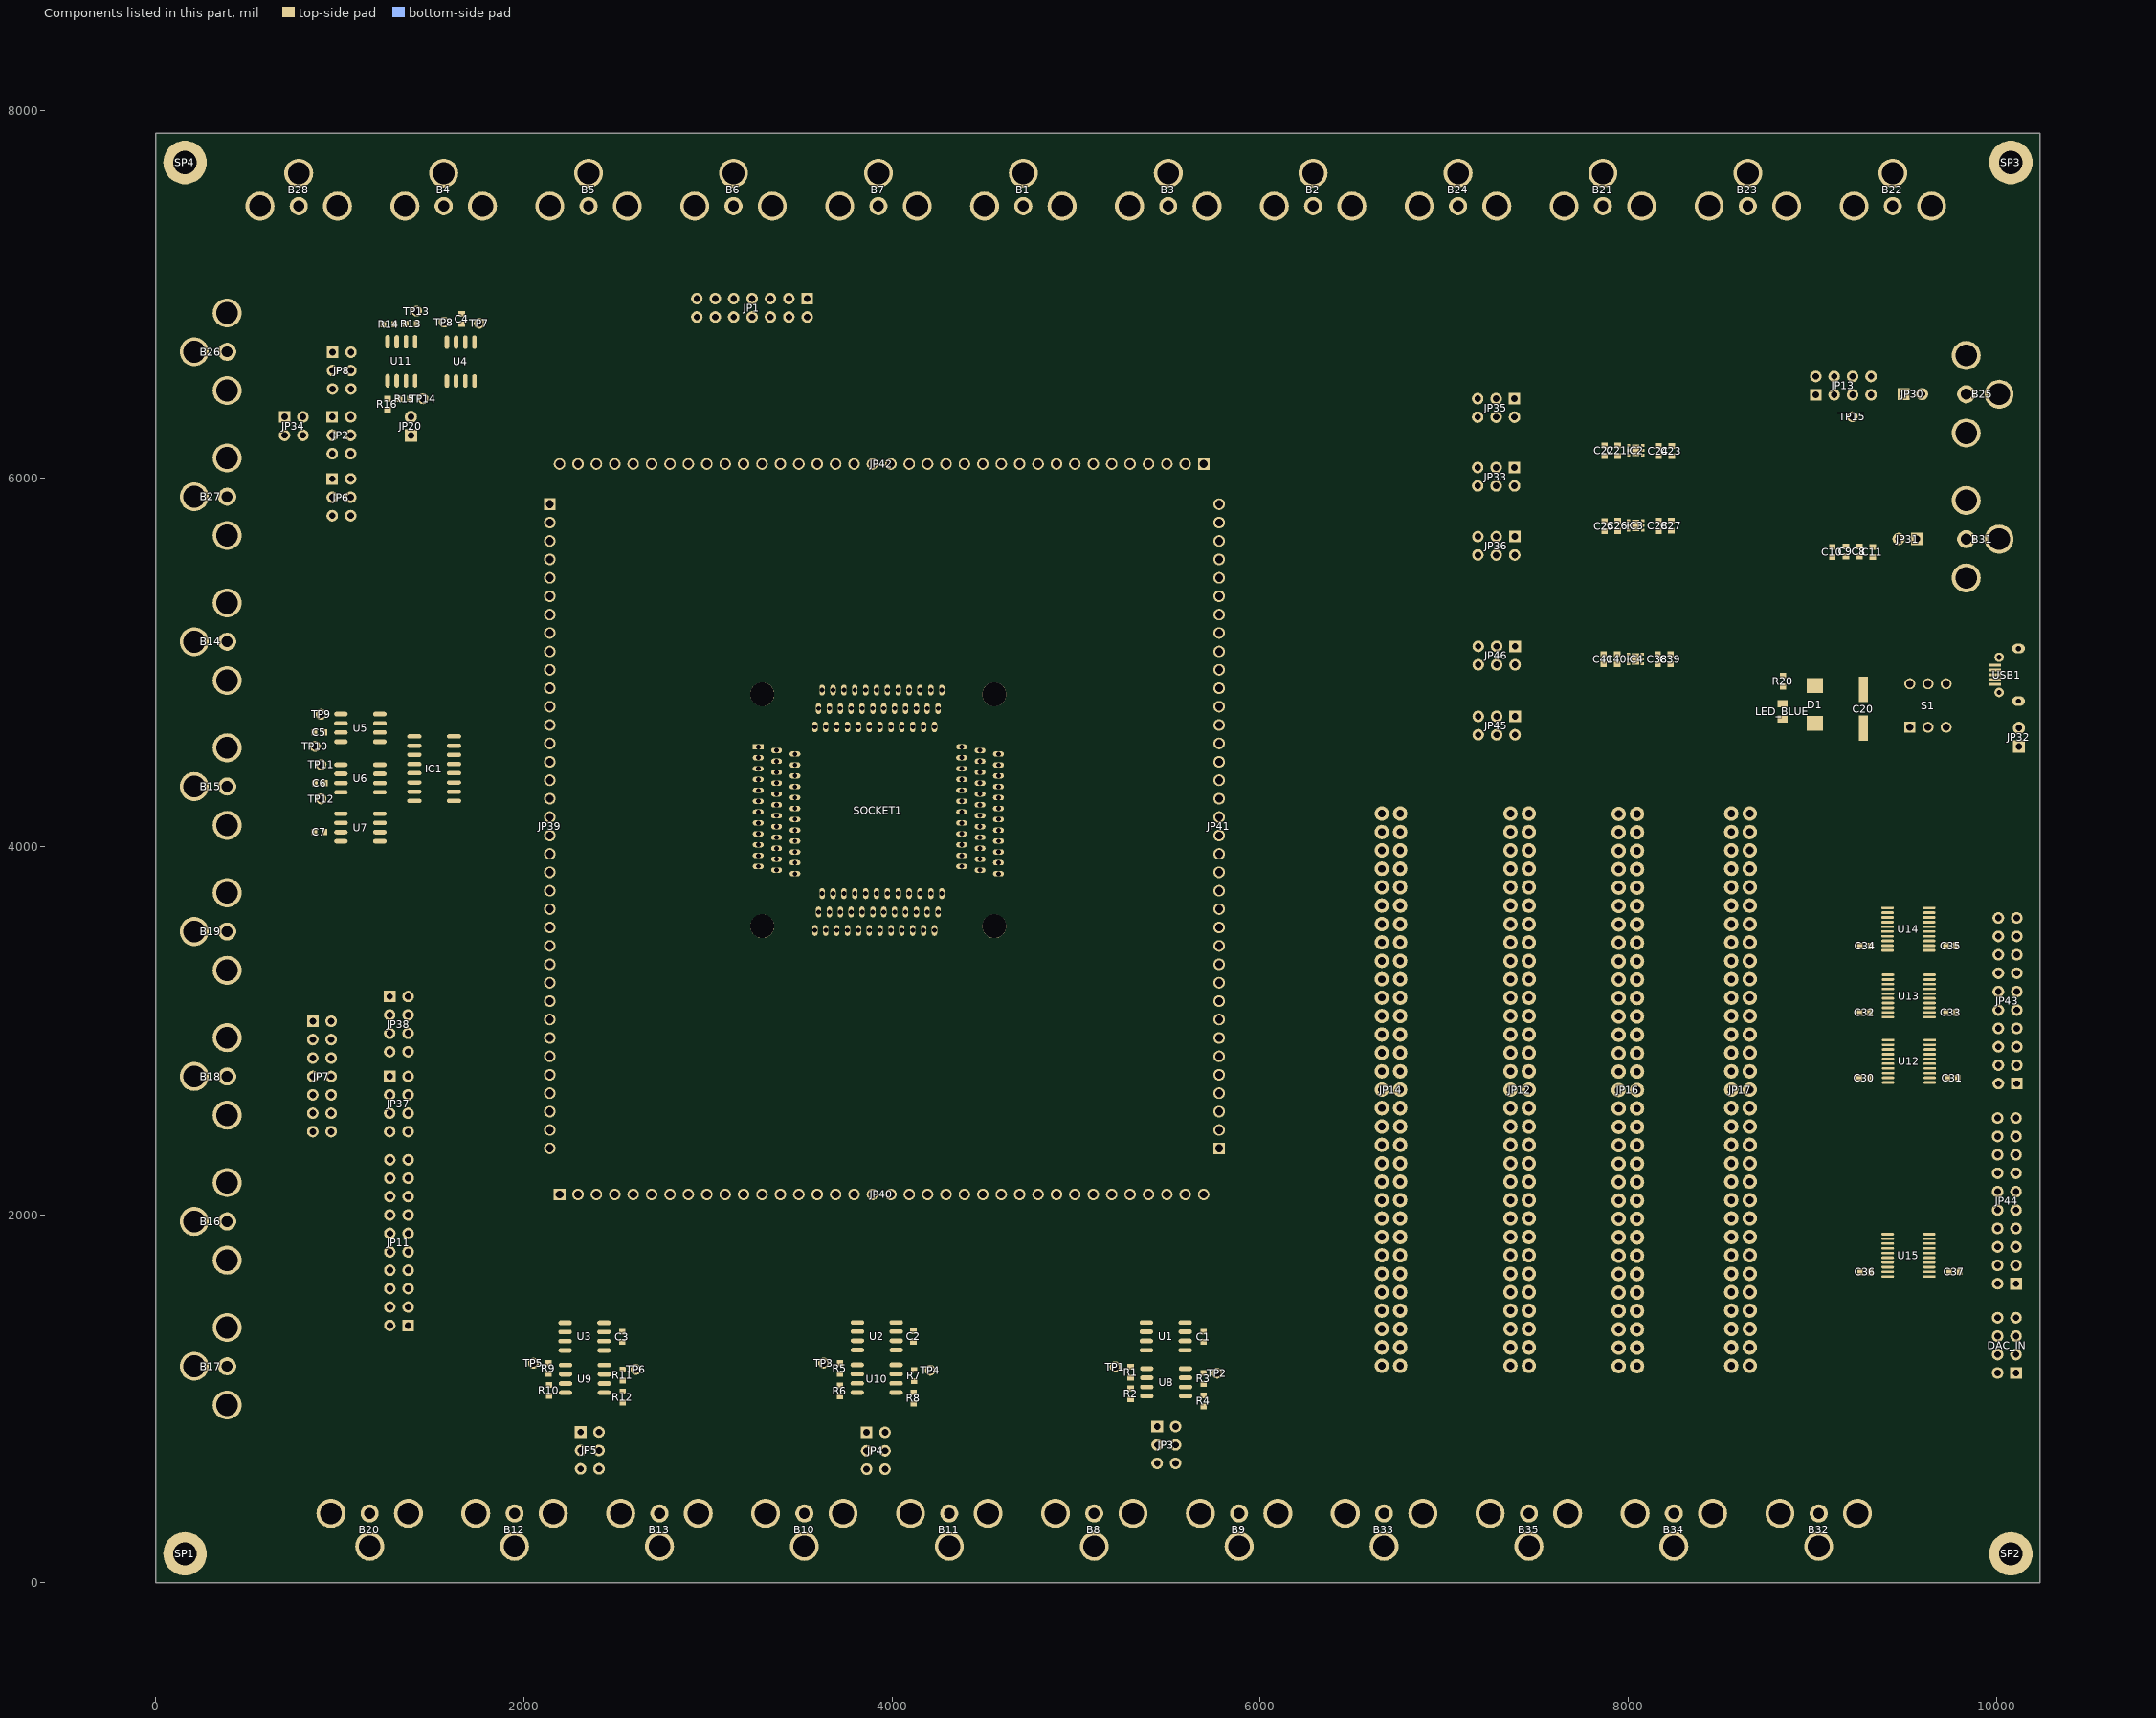
[diagram p0: the components of this part, seen from the top]
# Altium PCB MISC62794.PcbDoc (part 7 of 7)
Units mil, origin at the board's own origin, x right, y up, seen from the top; angles counter-clockwise.
Board outline 10236.22 x 7874.02 mil, 4 copper layers (Top Layer, GND, POWER, Bottom Layer); 158 components, 185 nets, 1211 pads, 1759 vias.

## Silkscreen, mask and mechanical layers (free items; w line width, h text height)
Top Overlay:
  text "VSSH" at 6229,7339 h50
  text "VBIT_PS_OUT2" at 7697,7338 h50
  text "VG_PS_OUT" at 9297,7336 h50
  text "VS_PS_OUT" at 8518,7335 h50
  text "VDD" at 3108,7334 h50
  text "VDDH" at 4647,7334 h50
  text "VDDC" at 5433,7334 h50
  text "VDD25" at 2297,7333 h50
  text "VBIT_PS_OUT1" at 6929,7328 h50
  text "VSS" at 3877,7317 h50
  text "VSSC" at 1511,7309 h50
  text "GND" at 730,7308 h50
  text "DAC14" at 782,6675 h40
  text "V25" at 528,6651 h50 r90
  text "GND" at 9233,6617 h40 r90
  text "GND" at 9132,6616 h40 r90
  text "GND" at 9334,6616 h40 r90
  text "GND" at 9028,6615 h40 r90
  text "FORMING" at 738,6570 h40
  text "GND" at 7245,6508 h40
  text "GND" at 7351,6507 h40
  text "GND" at 7145,6506 h40
  text "V25" at 832,6474 h40
  text "DCDC_OUT" at 9718,6332 h50 r90
  text "V25" at 1128,6311 h40
  text "V25" at 1209,6310 h40
  text "USB_5V" at 9032,6260 h40 r90
  text "USB_5V" at 9133,6257 h40 r90
  text "V11" at 7142,6242 h40
  text "V25" at 7247,6241 h40
  text "VCC5V" at 7346,6241 h40
  text "V11" at 1133,6219 h40
  text "V11" at 1234,6217 h40
  text "TEST" at 9233,6206 h40 r90
  text "DCDC_OUT" at 9333,6198 h40 r90
  text "VS1" at 3608,6169 h40 r90
  text "TSETDELAY_IN" at 3510,6168 h40 r90
  text "IREF" at 4006,6167 h40 r90
  text "TEST_PS_CTRL" at 3407,6166 h40 r90
  text "VSSC" at 3308,6165 h40 r90
  text "VLIM" at 3908,6165 h40 r90
  text "VS2" at 3712,6164 h40 r90
  text "VS_PS_OUT" at 4906,6164 h40 r90
  text "VDD" at 4408,6163 h40 r90
  text "VRES" at 3802,6162 h40 r90
  text "VSS" at 4304,6162 h40 r90
  text "VDDH" at 4604,6162 h40 r90
  text "VDDC" at 4709,6161 h40 r90
  text "VDDC" at 3204,6160 h40 r90
  text "VBIT_PS_OUT1" at 4109,6160 h40 r90
  text "VDD25" at 4505,6160 h40 r90
  text "NC" at 5706,6160 h40 r90
  text "VBIT_PS_OUT2" at 4207,6159 h40 r90
  text "VDDH" at 4806,6159 h40 r90
  text "CSB_ADD_1" at 5604,6156 h40 r90
  text "VDDH" at 3106,6155 h40 r90
  text "NC" at 2203,6154 h40 r90
  text "VBIT1" at 2402,6154 h40 r90
  text "VSSC" at 5208,6154 h40 r90
  text "CSB_ADD_4" at 5503,6153 h40 r90
  text "VSSH" at 2301,6152 h40 r90
  text "VBIT2" at 2508,6152 h40 r90
  text "VBIT_PS_CTRL" at 2806,6151 h40 r90
  text "VG_PS_CTRL" at 2905,6151 h40 r90
  text "VS_PS_CTRL" at 3006,6151 h40 r90
  text "CSB_ADD_2" at 5103,6150 h40 r90
  text "VG1" at 2606,6149 h40 r90
  text "CSB_ADD_0" at 5401,6149 h40 r90
  text "VG_PS_OUT" at 5011,6148 h40 r90
  text "VG2" at 2706,6147 h40 r90
  text "CSB_ADD_3" at 5303,6147 h40 r90
  text "GND" at 7245,6135 h40
  text "GND" at 7351,6134 h40
  text "GND" at 7145,6133 h40
  text "GND" at 1126,6118 h40
  text "GND" at 1222,6117 h40
  text "GND" at 821,5992 h40
  text "GND" at 1137,5991 h40
  text "GND" at 1138,5887 h40
  text "GND" at 816,5886 h40
  text "V11" at 523,5865 h50 r90
  text "V11" at 7145,5861 h40
  text "V25" at 7250,5860 h40
  text "VCC5V" at 7349,5860 h40
  text "NC" at 5924,5854 h40
  text "NC" at 1975,5851 h40
  text "NC" at 834,5786 h40
  text "NC" at 1143,5785 h40
  text "GND" at 7253,5757 h40
  text "GND" at 7359,5756 h40
  text "NC" at 1971,5755 h40
  text "GND" at 7153,5755 h40
  text "NC" at 5924,5747 h40
  text "NC" at 1967,5647 h40
  text "NC" at 5929,5646 h40
  text "VCC_5V" at 9711,5590 h50 r90
  text "NC" at 1966,5549 h40
  text "NC" at 5931,5546 h40
  text "V11" at 7147,5484 h40
  text "V25" at 7252,5483 h40
  text "VCC5V" at 7351,5483 h40
  text "NC" at 5934,5444 h40
  text "NC" at 1965,5443 h40
  text "NC" at 5938,5348 h40
  text "NC" at 1964,5347 h40
  text "Vbit_0" at 1903.04,5255 h40
  text "Vbit_16" at 5940.68,5248 h40
  text "GND" at 7254,5162 h40
  text "GND" at 7360,5161 h40
  text "GND" at 7154,5160 h40
  text "Vbit_1" at 1903.04,5150 h40
  text "Vbit_19" at 5940.6,5146 h40
  text "Vbit_2" at 1903.04,5055 h40
  text "VLIM" at 533,5054 h50 r90
  text "Vbit_17" at 5940.68,5049 h40
  text "Vbit_3" at 1903.04,4947 h40
  text "Vbit_22" at 5940.91,4946 h40
  text "3V3" at 7148,4887 h40
  text "3V3" at 7253,4886 h40
  text "VCC5V" at 7352,4886 h40
  text "Vbit_4" at 1903.04,4854 h40
  text "Vbit_20" at 5940.76,4849 h40
  text "GND" at 7249,4781 h40
  text "GND" at 7355,4780 h40
  text "GND" at 7149,4779 h40
  text "Vbit_5" at 1903.04,4751 h40
  text "Vbit_18" at 5940.6,4741 h40
  text "Vbit_6" at 1903.04,4653 h40
  text "Vbit_25" at 5940.48,4642 h40
  text "Vbit_7" at 1903.04,4556 h40
  text "Vbit_23" at 5940.68,4548 h40
  text "3V3" at 7156,4510 h40
  text "3V3" at 7261,4509 h40
  text "VCC5V" at 7360,4509 h40
  text "Vbit_8" at 1903.04,4454 h40
  text "Vbit_21" at 5945.59,4443 h40
  text "Vbit_9" at 1903.04,4357 h40
  text "VDDH" at 5961.94,4345 h40
  text "IREF" at 536,4268 h50 r90
  text "Vbit_10" at 1903.04,4251 h40
  text "Vbit_24" at 5940.76,4244 h40
  text "Vbit_16" at 6449,4184 h40
  text "VF3" at 7535,4174 h40
  text "VF1" at 8738,4174 h40
  text "Vbit_16" at 7148,4173 h40
  text "VF4" at 6831,4172 h40
  text "VF2" at 8130,4171 h40
  text "Vbit_16" at 7750,4167 h40
  text "Vbit_16" at 8358,4162 h40
  text "Vbit_11" at 1903.04,4154 h40
  text "VDDC" at 5960.45,4146 h40
  text "Vbit_19" at 6449,4078 h40
  text "VF3" at 7535,4072 h40
  text "Vbit_19" at 7148,4067 h40
  text "VF4" at 6831,4066 h40
  text "VF2" at 8129,4065 h40
  text "VF1" at 8738,4065 h40
  text "Vbit_19" at 7750,4061 h40
  text "Vbit_19" at 8358,4056 h40
  text "Vbit_12" at 1903.04,4053 h40
  text "VSSH" at 5965.84,4048 h40
  text "Vbit_17" at 6449,3979 h40
  text "VF1" at 8738,3972 h40
  text "VF3" at 7535,3971 h40
  text "VF4" at 6831,3970 h40
  text "VF2" at 8132,3969 h40
  text "Vbit_17" at 7148,3968 h40
  text "Vbit_17" at 7750,3962 h40
  text "Vbit_17" at 8358,3957 h40
  text "VSSC" at 1903.04,3951 h40
  text "VSSC" at 5964.35,3945 h40
  text "Vbit_22" at 6449,3878 h40
  text "VF3" at 7535,3871 h40
  text "Vbit_22" at 7148,3867 h40
  text "VF4" at 6831,3866 h40
  text "VF2" at 8133,3865 h40
  text "VF1" at 8738,3864 h40
  text "Vbit_22" at 7750,3861 h40
  text "Vbit_22" at 8358,3856 h40
  text "VSSH" at 1903.04,3852 h40
  text "Vbit_26" at 5940.68,3848 h40
  text "VF3" at 7535,3777 h40
  text "Vbit_20" at 6449,3775 h40
  text "VF1" at 8738,3768 h40
  text "VF4" at 6831,3767 h40
  text "Vbit_20" at 7148,3764 h40
  text "VF2" at 8134,3764 h40
  text "Vbit_20" at 7750,3758 h40
  text "VDDC" at 1903.04,3753 h40
  text "Vbit_20" at 8358,3753 h40
  text "Vbit_27" at 5940.68,3749 h40
  text "Vbit_18" at 6449,3672 h40
  text "VF2" at 8136,3670 h40
  text "VF4" at 6831,3668 h40
  text "VF3" at 7535,3666 h40
  text "VF1" at 8738,3665 h40
  text "Vbit_18" at 7148,3661 h40
  text "Vbit_18" at 7750,3655 h40
  text "Vbit_18" at 8358,3650 h40
  text "Vbit_14" at 1903.04,3647 h40
  text "Vbit_28" at 5940.6,3645 h40
  text "VG5" at 9798,3604 h40
  text "VG4" at 9879,3601 h40
  text "VF3" at 7542,3574 h40
  text "VF1" at 8737,3570 h40
  text "Vbit_25" at 6449,3569 h40
  text "VF4" at 6832,3568 h40
  text "VF2" at 8135,3564 h40
  text "Vbit_25" at 7148,3558 h40
  text "Vbit_25" at 7750,3552 h40
  text "Vbit_25" at 8358,3547 h40
  text "Vbit_29" at 5940.6,3546 h40
  text "VDDH" at 1903.04,3544 h40
  text "VG2" at 9880,3506 h40
  text "VG3" at 9797,3505 h40
  text "VRES" at 541,3491 h50 r90
  text "VF3" at 7542,3472 h40
  text "Vbit_23" at 6449,3470 h40
  text "VF2" at 8138,3468 h40
  text "VF4" at 6832,3462 h40
  text "VF1" at 8737,3461 h40
  text "Vbit_23" at 7148,3459 h40
  text "Vbit_23" at 7750,3453 h40
  text "Vbit_23" at 8358,3448 h40
  text "Vs_Sel_1" at 1903.04,3447 h40
  text "Vbit_30" at 5940.76,3446 h40
  text "VG0" at 9876,3403 h40
  text "VG1" at 9796,3401 h40
  text "Vbit_21" at 6449,3372 h40
  text "VF3" at 7542,3371 h40
  text "VF1" at 8737,3368 h40
  text "VF4" at 6832,3366 h40
  text "VF2" at 8139,3364 h40
  text "Vbit_21" at 7148,3361 h40
  text "Vbit_21" at 7750,3355 h40
  text "READ_EN" at 5897,3351 h40
  text "Vbit_21" at 8358,3350 h40
  text "WL_TEST" at 1903,3343 h40
  text "VS4" at 9882,3312 h40
  text "VS5" at 9797,3307 h40
  text "Vbit_24" at 6449,3271 h40
  text "VF3" at 7542,3271 h40
  text "STROBE" at 5916.7,3263 h40
  text "VF2" at 8140,3263 h40
  text "VF4" at 6832,3262 h40
  text "Vbit_24" at 7148,3260 h40
  text "VF1" at 8737,3260 h40
  text "Vbit_24" at 7750,3254 h40
  text "Vbit_13" at 1903.04,3250 h40
  text "Vbit_24" at 8358,3249 h40
  text "VS2" at 9884,3212 h40
  text "VS3" at 9793,3208 h40
  text "GND" at 1551,3180 h40
  text "VF3" at 7542,3177 h40
  text "V11" at 1446,3175 h40
  text "Vbit_26" at 6449,3170 h40
  text "VF1" at 8737,3164 h40
  text "VF4" at 6832,3163 h40
  text "Vbit_26" at 7148,3159 h40
  text "VF2" at 8140,3154 h40
  text "Vbit_26" at 7750,3153 h40
  text "Vbit_26" at 8358,3148 h40
  text "OEN" at 5987.36,3147 h40
  text "Vs_Sel_2" at 1903.04,3144 h40
  text "VS1" at 9815,3099 h40
  text "VS0" at 9889,3099 h40
  text "GND" at 1555,3077 h40
  text "Vbit_27" at 6449,3077 h40
  text "VLIM" at 1440,3074 h40
  text "Vbit_27" at 7148,3066 h40
  text "VF3" at 7542,3066 h40
  text "VF4" at 6832,3064 h40
  text "VF1" at 8737,3061 h40
  text "Vbit_27" at 7750,3060 h40
  text "Vbit_27" at 8358,3055 h40
  text "STATE_1" at 5913.34,3054 h40
  text "Vs_Sel_0" at 1903.04,3052 h40
  text "VF2" at 8139,3048 h40
  text "VLIM" at 691,3045 h40
  text "DAC7" at 1021,3043 h40
  text "STATE1" at 9815,2992 h40
  text "STATE2" at 9664,2991 h40
  text "GND" at 1558,2981 h40
  text "IREF" at 1446,2977 h40
  text "VF3" at 7546,2972 h40
  text "VF1" at 8735,2968 h40
  text "Vbit_28" at 6449,2965 h40
  text "VF4" at 6832,2965 h40
  text "Vbit_28" at 7148,2954 h40
  text "Vs_Sel_3" at 1903.04,2953 h40
  text "VF2" at 8142,2952 h40
  text "STATE_0" at 5908.51,2949 h40
  text "Vbit_28" at 7750,2948 h40
  text "IREF" at 706,2944 h40
  text "Vbit_28" at 8358,2943 h40
  text "DAC8" at 1017,2942 h40
  text "STATE0" at 9693,2903 h40
  text "ADD4" at 9853,2901 h40
  text "Vbit_29" at 6449,2882 h40
  text "GND" at 1558,2877 h40
  text "VREF" at 1448,2875 h40
  text "Vbit_29" at 7148,2871 h40
  text "VF3" at 7546,2870 h40
  text "Vbit_29" at 7750,2865 h40
  text "Vbit_29" at 8358,2860 h40
  text "VF4" at 6832,2859 h40
  text "VF1" at 8735,2859 h40
  text "NC" at 2004,2851 h40
  text "VF2" at 8143,2848 h40
  text "NC" at 5921,2847 h40
  text "DAC9" at 1020,2843 h40
  text "VRES" at 689,2838 h40
  text "ADD3" at 9695,2804 h40
  text "ADD2" at 9845,2803 h40
  text "Vbit_30" at 6449,2774 h40
  text "VF3" at 7546,2769 h40
  text "VF1" at 8735,2766 h40
  text "VF4" at 6832,2763 h40
  text "Vbit_30" at 7148,2763 h40
  text "NC" at 5921,2758 h40
  text "Vbit_30" at 7750,2757 h40
  text "Vbit_30" at 8358,2752 h40
  text "NC" at 2007,2751 h40
  text "VF2" at 8144,2747 h40
  text "GND" at 1614,2745 h40
  text "VS_PS" at 1441,2742 h40
  text "DAC10" at 1018,2741 h40
  text "VS_PS" at 675,2736 h40
  text "ADD0" at 9852,2672 h40
  text "ADD1" at 9711,2671 h40
  text "VF3" at 7546,2669 h40
  text "Vbit_0" at 6449,2663 h40
  text "NC" at 5918,2662 h40
  text "VF2" at 8146,2662 h40
  text "VF4" at 6832,2659 h40
  text "VF1" at 8735,2658 h40
  text "NC" at 2009,2655 h40
  text "Vbit_0" at 7148,2652 h40
  text "Vbit_0" at 7750,2646 h40
  text "DAC11" at 1020,2641 h40
  text "Vbit_0" at 8358,2641 h40
  text "VBIT_PS" at 1438,2639 h40
  text "GND" at 1616,2639 h40
  text "VBIT_PS" at 644,2636 h40
  text "VS_PS_CTRL" at 546,2603 h50 r90
  text "VF3" at 7546,2575 h40
  text "Vbit_1" at 6449,2567 h40
  text "VF1" at 8735,2562 h40
  text "VF4" at 6832,2560 h40
  text "NC" at 5918,2558 h40
  text "Vbit_1" at 7148,2556 h40
  text "VF2" at 8145,2556 h40
  text "NC" at 2010,2551 h40
  text "Vbit_1" at 7750,2550 h40
  text "Vbit_1" at 8358,2545 h40
  text "DAC12" at 1024,2544 h40
  text "GND" at 1611,2540 h40
  text "VG_PS" at 1446,2538 h40
  text "VG_PS" at 664,2534 h40
  text "NC" at 9823,2517 h40
  text "NC" at 9713,2515 h40
  text "Vbit_2" at 6449,2464 h40
  text "VF3" at 7546,2464 h40
  text "VF4" at 6832,2461 h40
  text "VF2" at 8148,2460 h40
  text "VF1" at 8735,2459 h40
  text "NC" at 5918,2454 h40
  text "Vbit_2" at 7148,2453 h40
  text "NC" at 2009,2448 h40
  text "Vbit_2" at 7750,2447 h40
  text "Vbit_2" at 8358,2442 h40
  text "TEST_PS" at 631,2440 h40
  text "DAC13" at 1022,2440 h40
  text "TEST_PS" at 1444,2437 h40
  text "GND" at 1622,2437 h40
  text "NC" at 9827,2415 h40
  text "NC" at 9715,2408 h40
  text "VF3" at 7551,2368 h40
  text "VF1" at 8734,2368 h40
  text "Vbit_3" at 6449,2364 h40
  text "VF4" at 6837,2363 h40
  text "VF2" at 8149,2356 h40
  text "Vbit_3" at 7148,2353 h40
  text "NC" at 5918,2351 h40
  text "NC" at 2012,2349 h40
  text "Vbit_3" at 7750,2347 h40
  text "Vbit_3" at 8358,2342 h40
  text "NC" at 9829,2320 h40
  text "NC" at 9714,2316 h40
  text "NC" at 1121,2295 h40
  text "NC" at 1476,2292 h40
  text "VF3" at 7551,2266 h40
  text "Vbit_4" at 6449,2261 h40
  text "VF1" at 8734,2259 h40
  text "VF4" at 6837,2257 h40
  text "VF2" at 8150,2255 h40
  text "Vbit_4" at 7148,2250 h40
  text "Vbit_4" at 7750,2244 h40
  text "Vbit_4" at 8358,2239 h40
  text "NC" at 9834,2219 h40
  text "NC" at 9719,2213 h40
  text "NC" at 1122,2186 h40
  text "NC" at 1479,2186 h40
  text "VF1" at 8734,2166 h40
  text "Vbit_5" at 6449,2165 h40
  text "VF3" at 7551,2165 h40
  text "VF4" at 6837,2161 h40
  text "Vbit_5" at 7148,2154 h40
  text "VF2" at 8149,2151 h40
  text "Vbit_5" at 7750,2148 h40
  text "Vbit_5" at 8358,2143 h40
  text "NC" at 9716,2122 h40
  text "IN_MCU" at 9810,2121 h40
  text "GND" at 1106,2087 h40
  text "OUT5" at 1458,2086 h40
  text "Vbit_6" at 6449,2068 h40
  text "VF3" at 7551,2065 h40
  text "VF1" at 8734,2058 h40
  text "VF4" at 6837,2057 h40
  text "Vbit_6" at 7148,2057 h40
  text "Vbit_6" at 7750,2051 h40
  text "Vbit_6" at 8358,2046 h40
  text "VF2" at 8148,2045 h40
  text "WL_TEST_MCU" at 9468,2015 h40
  text "OEN_MCU" at 9770,2015 h40
  text "GND" at 1108,1991 h40
  text "OUT7" at 1455,1985 h40
  text "NC" at 2209,1977 h40 r90
  text "VF3" at 7551,1971 h40
  text "VF1" at 8734,1962 h40
  text "Vbit_7" at 6449,1961 h40
  text "VF4" at 6837,1958 h40
  text "Vbit_7" at 7148,1950 h40
  text "VF2" at 8151,1949 h40
  text "Vbit_7" at 7750,1944 h40
  text "Vbit_7" at 8358,1939 h40
  text "STROBE_MCU" at 9702,1928 h40
  text "READ_EN_MCU" at 9409,1927 h40
  text "NC" at 5702,1917 h40 r90
  text "OUT_0" at 5004,1915 h40 r90
  text "VDDH" at 5599,1908 h40 r90
  text "VSSC" at 4104,1906 h40 r90
  text "OUT_3" at 4601,1904 h40 r90
  text "OUT_1" at 4203,1902 h40 r90
  text "VDDH" at 4308,1902 h40 r90
  text "VDDC" at 4404,1902 h40 r90
  text "VSS" at 4004,1901 h40 r90
  text "OUT_4" at 3803,1900 h40 r90
  text "VDD" at 3706,1899 h40 r90
  text "VDD25" at 5501,1898 h40 r90
  text "OUT_2" at 3899,1896 h40 r90
  text "VSSH" at 5399,1896 h40 r90
  text "OUT_6" at 3604,1895 h40 r90
  text "VSSC" at 3112,1893 h40 r90
  text "OUT_7" at 3501,1892 h40 r90
  text "OUT_5" at 3404,1891 h40 r90
  text "Vs_Sel_4" at 2305,1889 h40 r90
  text "Vs_Sel_5" at 2400,1889 h40 r90
  text "VDDC" at 3009,1887 h40 r90
  text "VSSH" at 3305,1887 h40 r90
  text "GND" at 1109,1886 h40
  text "VG_Sel_0" at 2506,1886 h40 r90
  text "VG_Sel_4" at 2903,1886 h40 r90
  text "STATE_2" at 5102,1885 h40 r90
  text "VG_Sel_1" at 2602,1883 h40 r90
  text "VG_Sel_2" at 2701,1883 h40 r90
  text "VG_Sel_3" at 2800,1883 h40 r90
  text "VG_Sel_5" at 3204,1883 h40 r90
  text "STATE_1" at 5201,1883 h40 r90
  text "OUT6" at 1457,1882 h40
  text "Vbit_8" at 6449,1869 h40
  text "VF3" at 7551,1860 h40
  text "VF4" at 6837,1859 h40
  text "VF1" at 8734,1859 h40
  text "Vbit_8" at 7148,1858 h40
  text "VBIT_Sel_2" at 4501,1853 h40 r90
  text "Vbit_8" at 7750,1852 h40
  text "VBIT_Sel_0" at 4698,1850 h40 r90
  text "VBIT_Sel_4" at 5302,1850 h40 r90
  text "Vbit_8" at 8358,1847 h40
  text "VBIT_Sel_5" at 4799,1846 h40 r90
  text "VBIT_Sel_3" at 4902,1846 h40 r90
  text "VF2" at 8152,1845 h40
  text "Vbit5" at 9739,1817 h40
  text "Vbit4" at 9862,1815 h40
  text "VBIT_PS_CTRL" at 551,1804 h50 r90
  text "GND" at 1112,1790 h40
  text "OUT4" at 1462,1787 h40
  text "VF3" at 7553,1773 h40
  text "Vbit_9" at 6449,1768 h40
  text "VF4" at 6830,1765 h40
  text "VF1" at 8737,1765 h40
  text "Vbit_9" at 7148,1757 h40
  text "Vbit_9" at 7750,1751 h40
  text "Vbit_9" at 8358,1746 h40
  text "VF2" at 8153,1744 h40
  text "Vbit3" at 9740,1735 h40
  text "Vbit2" at 9865,1732 h40
  text "GND" at 1110,1685 h40
  text "OUT2" at 1459,1685 h40
  text "VF3" at 7553,1671 h40
  text "Vbit_10" at 6449,1662 h40
  text "VF4" at 6830,1659 h40
  text "VF2" at 8155,1659 h40
  text "VF1" at 8737,1656 h40
  text "Vbit_10" at 7148,1651 h40
  text "Vbit_10" at 7750,1645 h40
  text "Vbit_10" at 8358,1640 h40
  text "Vbit1" at 9741,1608 h40
  text "Vbit0" at 9861,1608 h40
  text "GND" at 1110,1588 h40
  text "OUT1" at 1458,1584 h40
  text "VF3" at 7553,1570 h40
  text "Vbit_11" at 6449,1564 h40
  text "VF4" at 6830,1563 h40
  text "VF1" at 8737,1563 h40
  text "Vbit_11" at 7148,1553 h40
  text "VF2" at 8154,1553 h40
  text "Vbit_11" at 7750,1547 h40
  text "Vbit_11" at 8358,1542 h40
  text "GND" at 1113,1486 h40
  text "OUT3" at 1464,1481 h40
  text "VF3" at 7553,1470 h40
  text "Vbit_12" at 6449,1469 h40
  text "VF4" at 6830,1459 h40
  text "Vbit_12" at 7148,1458 h40
  text "VF2" at 8157,1457 h40
  text "VF1" at 8737,1455 h40
  text "Vbit_12" at 7750,1452 h40
  text "Vbit_12" at 8358,1447 h40
  text "RCLK" at 9829,1422 h40
  text "DIO" at 9696,1417 h40
  text "OUT0" at 1465,1382 h40
  text "GND" at 1101,1378 h40
  text "VF3" at 7553,1376 h40
  text "Vbit_13" at 6449,1364 h40
  text "VF4" at 6830,1360 h40
  text "VF1" at 8737,1359 h40
  text "Vbit_13" at 7148,1353 h40
  text "VF2" at 8158,1353 h40
  text "Vbit_13" at 7750,1347 h40
  text "Vbit_13" at 8358,1342 h40
  text "SCK" at 9689,1337 h40
  text "SPI_CLK" at 9794,1335 h40
  text "VF3" at 7547,1266 h40
  text "Vbit_14" at 6449,1265 h40
  text "VF1" at 8735,1262 h40
  text "VF4" at 6830,1261 h40
  text "Vbit_14" at 7148,1254 h40
  text "VF2" at 8159,1252 h40
  text "Vbit_14" at 7750,1248 h40
  text "Vbit_14" at 8358,1243 h40
  text "SPI_MISO" at 9775,1229 h40
  text "SPI_MOSI" at 9588,1227 h40
  text "Vbit_15" at 6449,1176 h40
  text "VF3" at 7544,1166 h40
  text "Vbit_15" at 7148,1165 h40
  text "VF1" at 8731,1164 h40
  text "VF2" at 8157,1163 h40
  text "VF4" at 6832,1160 h40
  text "Vbit_15" at 7750,1159 h40
  text "Vbit_15" at 8358,1154 h40
  text "GND" at 9674,1130 h40
  text "USB_5V" at 9800,1129 h40
  text "VG_PS_CTRL" at 561,1035 h50 r90
  text "DAC2" at 5609,839 h40
  text "DAC1" at 5276,837 h40
  text "DAC5" at 2144,811 h40
  text "DAC6" at 2473,808 h40
  text "DAC3" at 3703,805 h40
  text "DAC4" at 4030,805 h40
  text "VS2" at 5617,735 h40
  text "VS1" at 5295,728 h40
  text "VBIT2" at 2473,710 h40
  text "VBIT1" at 2141,707 h40
  text "VG1" at 3723,705 h40
  text "VG2" at 4028,705 h40
  text "GND" at 5618,631 h40
  text "GND" at 5289,630 h40
  text "GND" at 2154,611 h40
  text "GND" at 2480,607 h40
  text "GND" at 4026,601 h40
  text "GND" at 3714,600 h40
  text "TEST_PS_CTRL" at 1001,506 h50
  text "VF1" at 9003,482 h50
  text "VF4" at 6640,480 h50
  text "VF3" at 7419,480 h50
  text "VF2" at 8208,480 h50
  text "VG2" at 4268,477 h50
  text "VS1" at 5068,477 h50
  text "VBIT2" at 2674,475 h50
  text "VG1" at 3486,475 h50
  text "VBIT1" at 1888,472 h50
  text "VS2" at 5839,467 h50